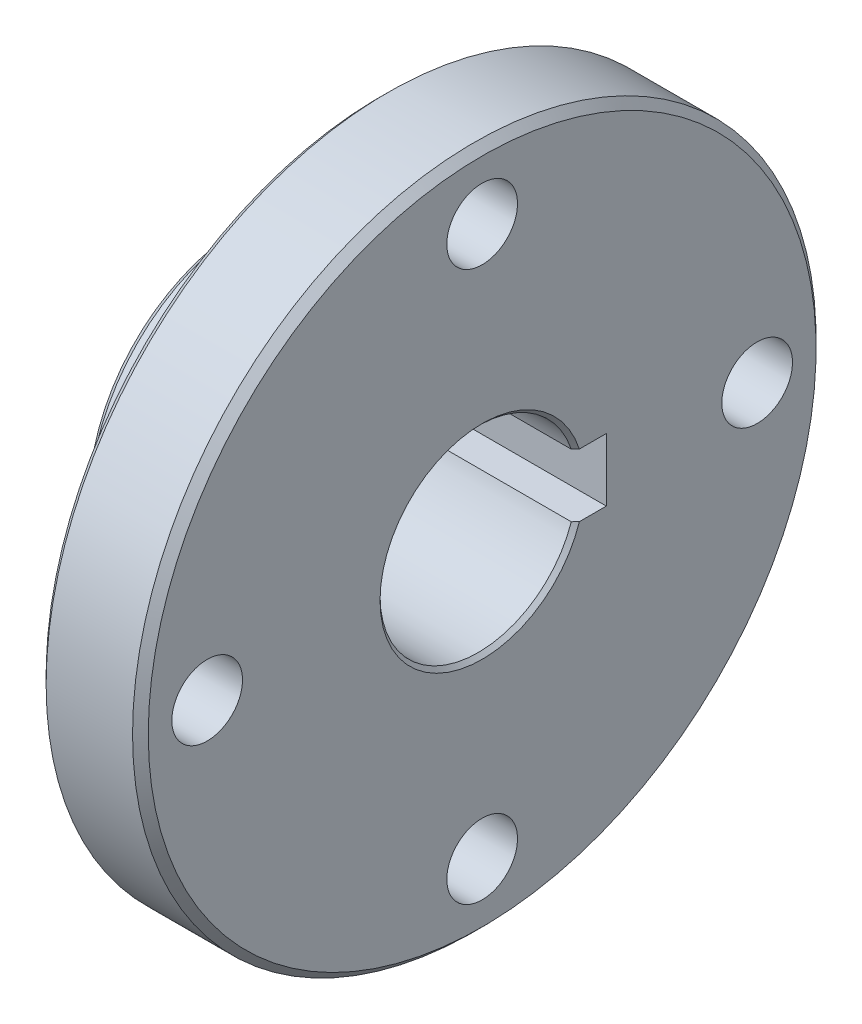
SolidWorks part; units mm, degrees
ref_plane "Front Plane" through (0, 0, 0) normal (0, 0, 1) x (1, 0, 0)
ref_plane "Top Plane" through (0, 0, 0) normal (0, 1, 0) x (1, 0, 0)
ref_plane "Right Plane" through (0, 0, 0) normal (1, 0, 0) x (0, 0, -1)
sketch "Sketch1" plane through (0, 0, 0) normal (0, 0, 1) x (1, 0, 0)
  line L0 (0, 12.5) -> (0, 21)
  line L1 (0, 21) -> (17, 21)
  line L2 (17, 21) -> (17, 43.5)
  line L3 (17, 43.5) -> (30, 43.5)
  line L4 (30, 43.5) -> (30, 12.5)
  line L5 (0, 12.5) -> (30, 12.5)
  line L6 (0, 0) -> (17, 0) construction
  dimension "D1" = 12.5
  dimension "D2" = 21
  dimension "D3" = 43.5
  dimension "D4" = 17
  dimension "D5" = 13
revolve "Revolve1" add sketch "Sketch1" angle 360 about L6
chamfer "Chamfer1" distance 1 angle 45 1 edges at (0, 0, 21)
chamfer "Chamfer2" distance 0.5 angle 45 2 edges at (30, 0, 12.5) (0, 0, 12.5)
fillet "Fillet1" radius 5 1 edges at (17, 0, 21)
chamfer "Chamfer3" distance 1 angle 45 2 edges at (30, 0, 43.5) (17, 0, 43.5)
sketch "Sketch2" plane through (17, 0, 0) normal (-1, 0, 0) x (0, 0, 1)
  line L0 (35, 0) -> (-39.3978, 0) construction
  line L1 (0, 35) -> (0, -39.2258) construction
  circle A0 centre (0, 0) radius 35 construction
  circle A1 centre (-35, 0) radius 4.5
  circle A2 centre (0, -35) radius 4.5
  circle A3 centre (0, 35) radius 4.5
  circle A4 centre (35, 0) radius 4.5
  dimension "D1" = 9
extrude "Cut-Extrude1" cut sketch "Sketch2" against normal blind 20
sketch "Sketch3" plane through (30, 0, 0) normal (1, 0, 0) x (0, 0, -1)
  line L1 (15.8, 4) -> (7.7419, 4)
  line L2 (15.8, 4) -> (15.8, -4)
  line L3 (15.8, -4) -> (7.7419, -4)
  line L4 (7.7419, 4) -> (7.7419, -4)
  dimension "D1" = 4
  dimension "D2" = 8
  dimension "D3" = 15.8
extrude "Cut-Extrude2" cut sketch "Sketch3" against normal through all
